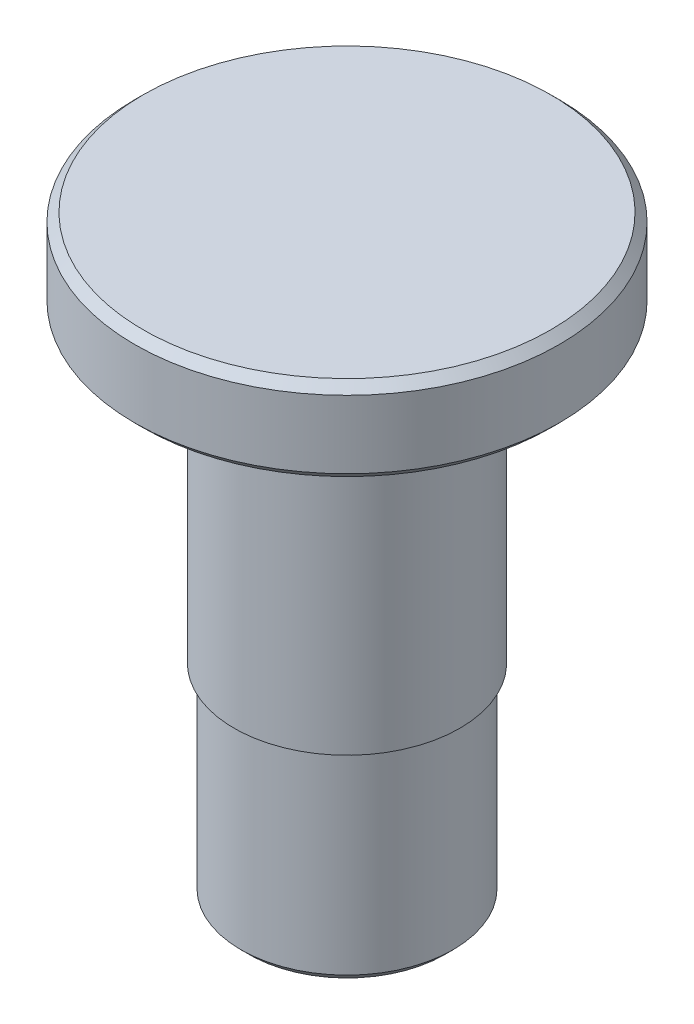
SolidWorks part; units mm, degrees
material "20#"
ref_plane "Front Plane" through (0, 0, 0) normal (0, 0, 1) x (1, 0, 0)
ref_plane "Top Plane" through (0, 0, 0) normal (0, 1, 0) x (1, 0, 0)
ref_plane "Right Plane" through (0, 0, 0) normal (1, 0, 0) x (0, 0, -1)
sketch "Sketch1" plane through (0, 0, 0) normal (0, 0, 1) x (1, 0, 0)
  line L1 (-139.2869, -435.6857) -> (-139.6869, -435.6857)
  line L2 (-139.6869, -417.6857) -> (-139.6869, -437.6857) construction
  line L3 (-139.6869, -435.6857) -> (-139.6869, -417.6857)
  line L4 (-139.6869, -417.6857) -> (-145.5369, -417.6857)
  line L5 (-145.5369, -417.6857) -> (-145.5369, -412.6857)
  line L6 (-145.5369, -412.6857) -> (-133.0369, -412.6857)
  line L9 (-133.0369, -412.6857) -> (-133.0369, -446.4007) construction
  line L10 (-139.2869, -435.6857) -> (-139.2869, -447.6857)
  line L11 (-139.2869, -447.6857) -> (-133.0369, -447.6857)
  line L12 (-139.2869, -437.6857) -> (-139.2869, -440.8857) construction
  line L13 (34.4631, -437.6857) -> (-150.5369, -437.6857) construction
  line L14 (-133.0369, -447.6857) -> (-133.0369, -412.6857)
  dimension "D1" = 6.65
  dimension "D2" = 2
  dimension "D3" = 12
  dimension "D4" = 5
  dimension "D5" = 12.5
revolve "Revolve1" add sketch "Sketch1" angle 360 about L9
chamfer "Chamfer1" distance 0.5 angle 45 3 edges at (-145.5369, -412.6857, 0) (-145.5369, -417.6857, 0) (-139.2869, -447.6857, 0)
